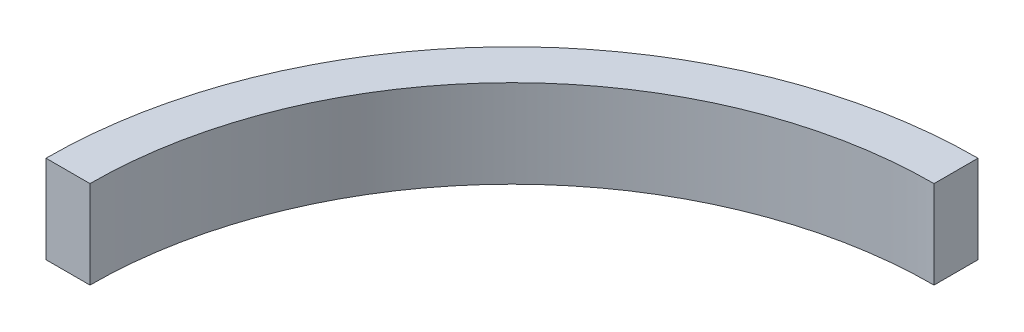
SolidWorks part; units mm, degrees
material "A3"
ref_plane "前视基准面" through (0, 0, 0) normal (0, 0, 1) x (1, 0, 0)
ref_plane "上视基准面" through (0, 0, 0) normal (0, 1, 0) x (1, 0, 0)
ref_plane "右视基准面" through (0, 0, 0) normal (1, 0, 0) x (0, 0, -1)
sketch "草图1" plane through (0, 0, 0) normal (0, 1, 0) x (1, 0, 0)
  line L0 (0, 144) -> (0, 0) construction
  line L1 (0, 0) -> (-144, 0) construction
  line L2 (-159, 0) -> (-144, 0)
  line L3 (0, 159) -> (0, 144)
  arc A0 (0, 144) -> (-144, 0) centre (0, 0) ccw
  arc A1 (0, 159) -> (-159, 0) centre (0, 0) ccw
  dimension "D1" = 288
  dimension "D2" = 15
extrude "凸台-拉伸1" add sketch "草图1" along normal blind 30
